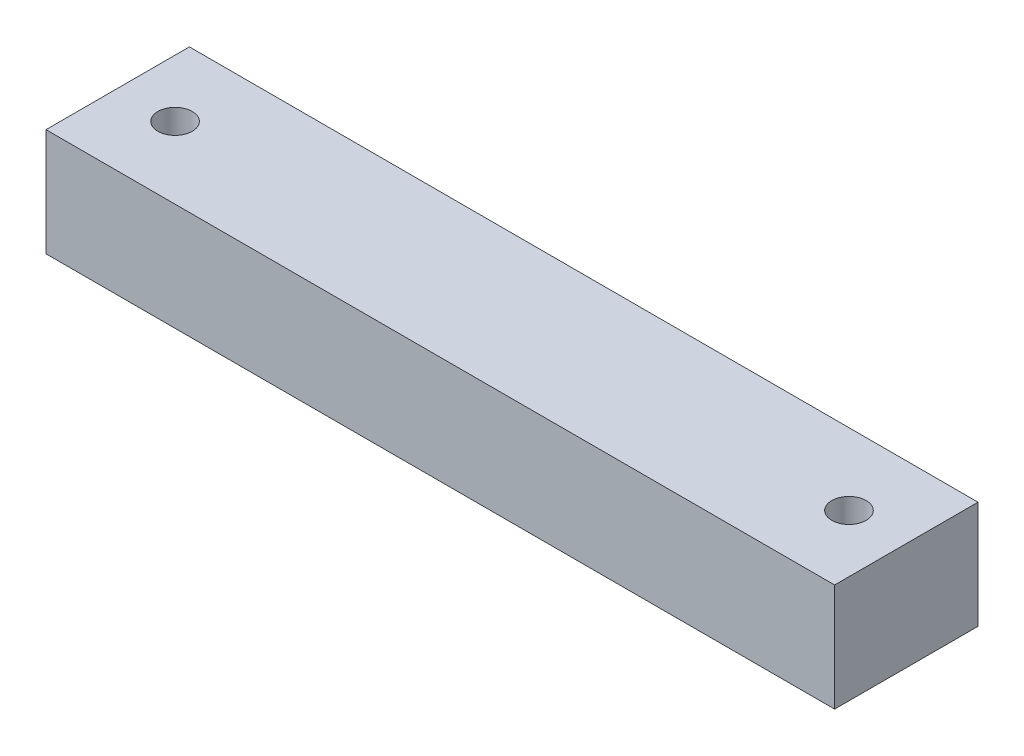
from build123d import *

# Parameters (mm, degrees)
SKETCH_1_W         = 110
SKETCH_1_H         = 20
EXTRUDE_1_DEPTH    = 15
HOLE_WIZARD_M4_1_D = 4.8


with BuildPart() as part:
    # 草图1 → 凸台-拉伸1 (new body)
    with BuildSketch(Plane(origin=(0, 0, 0), x_dir=(1, 0, 0), z_dir=(0, 1, 0))):
        Rectangle(SKETCH_1_W, SKETCH_1_H)
    extrude(amount=EXTRUDE_1_DEPTH)

    # M4 间隙孔1 (through all)
    with Locations(Plane(origin=(0, 15, 0), x_dir=(1, 0, 0), z_dir=(0, 1, 0))):
        with Locations((-47, 0), (47, 0)):
            Hole(HOLE_WIZARD_M4_1_D / 2)


solid = part.part
